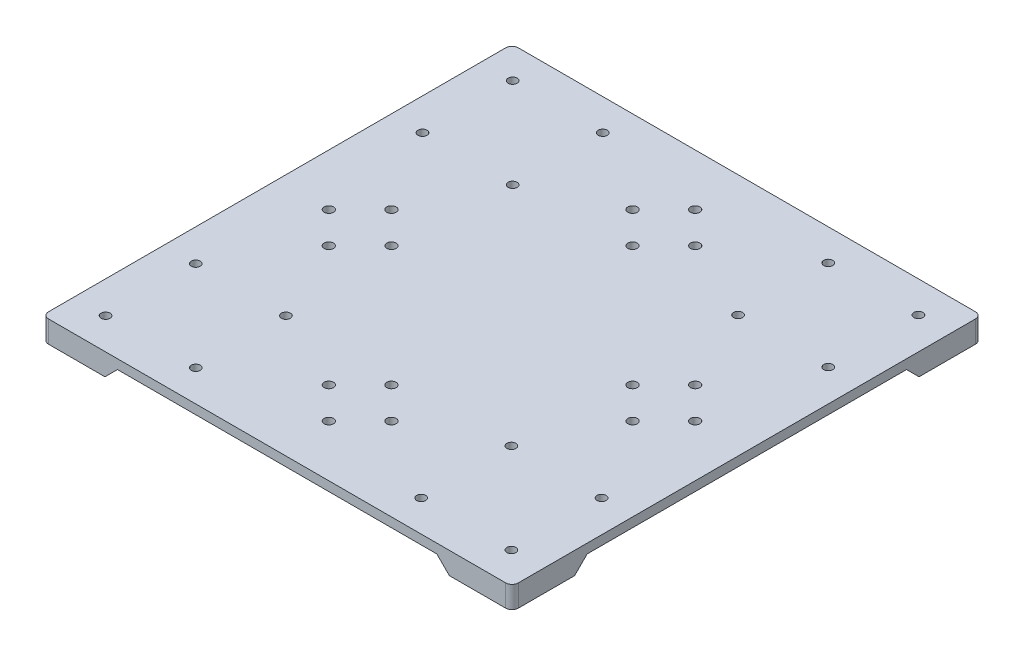
SolidWorks part; units mm, degrees
ref_plane "Front Plane" through (0, 0, 0) normal (0, 0, 1) x (1, 0, 0)
ref_plane "Top Plane" through (0, 0, 0) normal (0, 1, 0) x (1, 0, 0)
ref_plane "Right Plane" through (0, 0, 0) normal (1, 0, 0) x (0, 0, -1)
other "Configuration Table"
sketch "Sketch1" plane through (0, 0, 0) normal (0, 1, 0) x (1, 0, 0)
  line L1 (-75, -75) -> (75, -75)
  line L2 (-75, -75) -> (-75, 75)
  line L3 (-75, 75) -> (75, 75)
  line L4 (75, -75) -> (75, 75)
  line L5 (-75, -75) -> (75, 75) construction
  line L6 (-75, 75) -> (75, -75) construction
  point P0 (0, 0)
  dimension "D1" = 150
extrude "Boss-Extrude1" add sketch "Sketch1" along normal blind 3
sketch "Sketch2" plane through (0, 3, 0) normal (0, 1, 0) x (1, 0, 0)
  line L0 (-82.5623, 0) -> (98.2295, 0) construction
  line L1 (0, 86.5822) -> (0, -88.3138) construction
  line L3 (75, 75) -> (-75, 75) construction
  line L7 (-66.5, 34.5) -> (-30.5, 34.5)
  line L8 (-66.5, 34.5) -> (-66.5, 70.5)
  line L9 (-66.5, 70.5) -> (-30.5, 70.5)
  line L10 (-30.5, 34.5) -> (-30.5, 70.5)
  line L11 (-66.5, 34.5) -> (-30.5, 70.5) construction
  line L12 (-66.5, 70.5) -> (-30.5, 34.5) construction
  circle A0 centre (-64.8, 65) radius 1.44
  circle A1 centre (-36, 65) radius 1.44
  circle A2 centre (-64.8, 36.2) radius 1.44
  circle A3 centre (-36, 36.2) radius 1.44
  circle A4 centre (36, 65) radius 1.44
  circle A5 centre (64.8, 65) radius 1.44
  circle A6 centre (64.8, 36.2) radius 1.44
  circle A7 centre (36, 36.2) radius 1.44
  circle A8 centre (-64.8, -36.2) radius 1.44
  circle A9 centre (-64.8, -65) radius 1.44
  circle A10 centre (-36, -65) radius 1.44
  circle A11 centre (-36, -36.2) radius 1.44
  circle A12 centre (64.8, -65) radius 1.44
  circle A13 centre (36, -65) radius 1.44
  circle A14 centre (36, -36.2) radius 1.44
  circle A15 centre (64.8, -36.2) radius 1.44
  point P13 (-48.5, 52.5)
  point P14 (-48.5, 52.5)
  dimension "D1" = 2.88
  dimension "D2" = 28.8
  dimension "D3" = 28.8
  dimension "D7" = 10
extrude "Cut-Extrude1" cut sketch "Sketch2" against normal through all contours A11 | A8 | A9 | A10 | A14 | A13 | A15 | A12 | A6 | A5 | A4 | A7 | A1 | A3 | A2 | A0
sketch "Sketch3" plane through (0, 3, 0) normal (0, 1, 0) x (1, 0, 0)
  line L0 (-75, 0) -> (75, 0) construction
  line L1 (-75, 75) -> (-75, -75) construction
  line L2 (75, -75) -> (75, 75) construction
  line L3 (0, 75) -> (0, -75) construction
  line L4 (75, 75) -> (-75, 75) construction
  line L5 (-75, -75) -> (75, -75) construction
  line L6 (-36, 65) -> (-64.8, 36.2)
  line L7 (-64.8, 65) -> (-36, 36.2)
  circle A0 centre (-48.5, 0) radius 12.5
  circle A1 centre (-48.5, 0) radius 7.5
  circle A2 centre (-38.5, 0) radius 1.5
  circle A3 centre (-48.5, 10) radius 1.5
  circle A4 centre (-58.5, 0) radius 1.5
  circle A5 centre (-48.5, -10) radius 1.5
  circle A6 centre (0, 0) radius 22.0858 construction
  circle A7 centre (0, 48.5) radius 12.5
  circle A8 centre (0, 48.5) radius 7.5
  circle A9 centre (0, 38.5) radius 1.5
  circle A10 centre (10, 48.5) radius 1.5
  circle A11 centre (0, 58.5) radius 1.5
  circle A12 centre (-10, 48.5) radius 1.5
  circle A13 centre (48.5, 0) radius 12.5
  circle A14 centre (48.5, 0) radius 7.5
  circle A15 centre (38.5, 0) radius 1.5
  circle A16 centre (48.5, -10) radius 1.5
  circle A17 centre (58.5, 0) radius 1.5
  circle A18 centre (48.5, 10) radius 1.5
  circle A19 centre (0, -48.5) radius 12.5
  circle A20 centre (0, -48.5) radius 7.5
  circle A21 centre (0, -38.5) radius 1.5
  circle A22 centre (-10, -48.5) radius 1.5
  circle A23 centre (0, -58.5) radius 1.5
  circle A24 centre (10, -48.5) radius 1.5
  point P20 (-50.4, 50.6)
  point P71 (0, 0)
  dimension "D1" = 25
  dimension "D2" = 15
  dimension "D3" = 10
  dimension "D4" = 3
  dimension "D5" = 10
  dimension "D8" = 4
  dimension "D6" = 10
  dimension "D7" = 10
extrude "Cut-Extrude2" cut sketch "Sketch3" against normal through all contours A2 | A3 | A4 | A5 | A22 | A23 | A24 | A21 | A17 | A18 | A15 | A9 | A10 | A11 | A12 | A16
fillet "Fillet1" radius 2 4 edges at (-75, 1.5, -75) (75, 1.5, -75) (75, 1.5, 75) (-75, 1.5, 75)
sketch "Sketch4" plane through (0, 0, 0) normal (0, -1, 0) x (1, 0, 0)
  line L0 (73, -75) -> (-73, -75) construction
  line L1 (75, 73) -> (75, -73) construction
  line L2 (-75, -73) -> (-75, 73) construction
  line L3 (-73, 75) -> (73, 75) construction
  line L4 (73, -75) -> (-73, -75)
  line L5 (75, 73) -> (75, -73)
  line L6 (-75, -73) -> (-75, 73)
  line L7 (-73, 75) -> (73, 75)
  line L8 (-72, 72) -> (72, 72)
  line L9 (72, 72) -> (72, -72)
  line L10 (72, -72) -> (-72, -72)
  line L11 (-72, -72) -> (-72, 72)
  arc A0 (-75, -73) -> (-73, -75) centre (-73, -73) ccw construction
  arc A1 (73, -75) -> (75, -73) centre (73, -73) ccw construction
  arc A2 (75, 73) -> (73, 75) centre (73, 73) ccw construction
  arc A3 (-73, 75) -> (-75, 73) centre (-73, 73) ccw construction
  arc A4 (-75, -73) -> (-73, -75) centre (-73, -73) ccw
  arc A5 (73, -75) -> (75, -73) centre (73, -73) ccw
  arc A6 (75, 73) -> (73, 75) centre (73, 73) ccw
  arc A7 (-73, 75) -> (-75, 73) centre (-73, 73) ccw
  arc A8 (72, 72) -> (72, 72) centre (72, 72) ccw
  arc A9 (72, -72) -> (72, -72) centre (72, -72) ccw
  arc A10 (-72, -72) -> (-72, -72) centre (-72, -72) ccw
  arc A11 (-72, 72) -> (-72, 72) centre (-72, 72) ccw
  dimension "D1" = 3
extrude "Boss-Extrude2" add sketch "Sketch4" along normal blind 4
sketch "Sketch5" plane through (0, 0, 75) normal (0, 0, 1) x (1, 0, 0)
  line L0 (0, 13.3588) -> (0, -11.9693) construction
  line L1 (-55, -4) -> (-51, 0)
  line L2 (73, -4) -> (-73, -4) construction
  line L3 (-51, 0) -> (51, 0)
  line L4 (55, -4) -> (51, 0)
  line L5 (-55, -4) -> (55, -4)
  point P10 (0, 0)
  dimension "D1" = 45
  dimension "D2" = 55
extrude "Cut-Extrude3" cut sketch "Sketch5" against normal through all
sketch "Sketch6" plane through (-75, 0, 0) normal (-1, 0, 0) x (0, 0, 1)
  line L0 (0, 13.8023) -> (0, -11.5258) construction
  line L1 (-55, -4) -> (-51, 0)
  line L2 (-51, 0) -> (51, 0)
  line L3 (55, -4) -> (51, 0)
  line L4 (-55, -4) -> (55, -4)
  line L5 (73, -4) -> (-73, -4) construction
  point P6 (0, 0)
  dimension "D1" = 55
  dimension "D2" = 45
extrude "Cut-Extrude4" cut sketch "Sketch6" against normal through all
